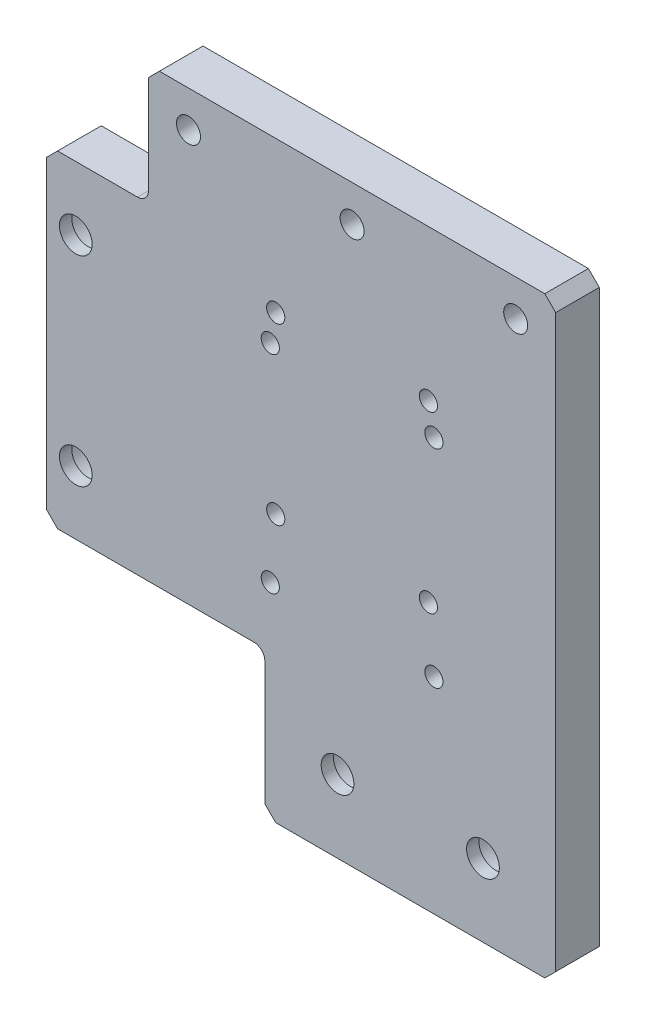
from build123d import *

# Parameters (mm, degrees)
SKETCH_1_W                   = 140
SKETCH_1_H                   = 90
EXTRUDE_1_DEPTH              = 6
HOLE_WIZARD_M6_2_D           = 5
PATTERN_LINEAR_3_COUNT       = 2
PATTERN_LINEAR_3_PITCH       = 45
PATTERN_LINEAR_3_COPY_1_D    = 5
HOLE_WIZARD_M8_1_D           = 9
HOLE_WIZARD_M8_1_CBORE_D     = 15
HOLE_WIZARD_M8_1_CBORE_DEPTH = 8.6
SKETCH_11_W                  = 112
SKETCH_11_H                  = 12
EXTRUDE_2_DEPTH              = 33
FILLET_1_R                   = 3
CHAMFER_2_SIZE               = 3
HOLE_WIZARD_M6_1_D           = 6.6
HOLE_WIZARD_M6_1_DEPTH       = 15
HOLE_WIZARD_M6_1_CBORE_D     = 11
HOLE_WIZARD_M6_1_CBORE_DEPTH = 6.4
HOLE_WIZARD_M6_1_TIP         = 1.982840043
HOLE_WIZARD_M6_3_D           = 5
SKETCH_16_W                  = 80
SKETCH_16_H                  = 43
EXTRUDE_3_DEPTH              = 12
CHAMFER_3_SIZE               = 3
FILLET_2_R                   = 3
HOLE_WIZARD_M8_2_D           = 9
HOLE_WIZARD_M8_2_CBORE_D     = 15
HOLE_WIZARD_M8_2_CBORE_DEPTH = 8.6


with BuildPart() as part:
    # 草图1 → 凸台-拉伸1 (new, symmetric)
    with BuildSketch(Plane.XY):
        Rectangle(SKETCH_1_W, SKETCH_1_H)
    extrude(amount=EXTRUDE_1_DEPTH, both=True)

    # M6 螺纹孔2 (through all)
    with Locations(Plane.XY.offset(6)):
        with Locations((36.5, 28.5)):
            hole_wizard_m6_2 = Hole(HOLE_WIZARD_M6_2_D / 2)

    # 镜向1: M6 螺纹孔2 across plane
    add(hole_wizard_m6_2.mirror(Plane.ZX), mode=Mode.SUBTRACT)

    # 阵列(线性)3: M6 螺纹孔2 ×2
    with Locations(*[(-i * PATTERN_LINEAR_3_PITCH, 0, 0) for i in range(1, PATTERN_LINEAR_3_COUNT)]):
        add(hole_wizard_m6_2, mode=Mode.SUBTRACT)

    # 阵列(线性)3 copy 1 (through all)
    with Locations(Plane(origin=(-45, 0, 6), x_dir=(1, 0, 0), z_dir=(0, 0, 1))):
        with Locations((36.5, -28.5)):
            Hole(PATTERN_LINEAR_3_COPY_1_D / 2)

    # M8 六角凹头螺钉的柱形沉头孔1 (through all)
    with Locations(Plane(origin=(0, 0, -6), x_dir=(-1, 0, 0), z_dir=(0, 0, -1))):
        with Locations((62, 27.5), (62, -27.5)):
            CounterBoreHole(HOLE_WIZARD_M8_1_D / 2, HOLE_WIZARD_M8_1_CBORE_D / 2, HOLE_WIZARD_M8_1_CBORE_DEPTH)

    # 草图11 → 凸台-拉伸2 (add)
    with BuildSketch(Plane(origin=(0, 45, 0), x_dir=(1, 0, 0), z_dir=(0, 1, 0))):
        with Locations((14, 0)):
            Rectangle(SKETCH_11_W, SKETCH_11_H)
    extrude(amount=EXTRUDE_2_DEPTH)

    # 圆角1
    fillet_1_edges = [part.edges().sort_by_distance(p)[0] for p in [
        (-42, 45, 0),
    ]]
    fillet(fillet_1_edges, radius=FILLET_1_R)

    # 倒角2
    chamfer_2_edges = [part.edges().sort_by_distance(p)[0] for p in [
        (70, -45, 0),
        (-70, -45, 0),
        (-70, 45, 0),
        (-42, 78, 0),
        (70, 78, 0),
    ]]
    chamfer(chamfer_2_edges, length=CHAMFER_2_SIZE)

    # M6 六角凹头螺钉的柱形沉头孔1
    with Locations(Plane(origin=(0, 0, -6), x_dir=(-1, 0, 0), z_dir=(0, 0, -1))):
        with Locations((-59, 68), (-14, 68), (31, 68)):
            CounterBoreHole(HOLE_WIZARD_M6_1_D / 2, HOLE_WIZARD_M6_1_CBORE_D / 2, HOLE_WIZARD_M6_1_CBORE_DEPTH, depth=HOLE_WIZARD_M6_1_DEPTH)
            with Locations((0, 0, -(HOLE_WIZARD_M6_1_DEPTH + HOLE_WIZARD_M6_1_TIP / 2))):  # 118° drill point
                Cone(0, HOLE_WIZARD_M6_1_D / 2, HOLE_WIZARD_M6_1_TIP, mode=Mode.SUBTRACT)

    # M6 螺纹孔3 (through all)
    with Locations(Plane(origin=(0, 0, -6), x_dir=(-1, 0, 0), z_dir=(0, 0, -1))):
        with Locations((7, 36.5), (-35, 36.5), (7, -11.5), (-35, -11.5)):
            Hole(HOLE_WIZARD_M6_3_D / 2)

    # 草图16 → 凸台-拉伸3 (add)
    with BuildSketch(Plane(origin=(0, 0, -6), x_dir=(-1, 0, 0), z_dir=(0, 0, -1))):
        with Locations((-30, -63.5)):
            Rectangle(SKETCH_16_W, SKETCH_16_H)
    extrude(amount=-EXTRUDE_3_DEPTH)

    # 倒角3
    chamfer_3_edges = [part.edges().sort_by_distance(p)[0] for p in [
        (70, -85, 0),
        (-10, -85, 0),
    ]]
    chamfer(chamfer_3_edges, length=CHAMFER_3_SIZE)

    # 圆角2
    fillet_2_edges = [part.edges().sort_by_distance(p)[0] for p in [
        (-10, -45, 0),
    ]]
    fillet(fillet_2_edges, radius=FILLET_2_R)

    # M8 六角凹头螺钉的柱形沉头孔2 (through all)
    with Locations(Plane(origin=(0, 0, -6), x_dir=(-1, 0, 0), z_dir=(0, 0, -1))):
        with Locations((-50, -65), (-10, -65)):
            CounterBoreHole(HOLE_WIZARD_M8_2_D / 2, HOLE_WIZARD_M8_2_CBORE_D / 2, HOLE_WIZARD_M8_2_CBORE_DEPTH)


solid = part.part
